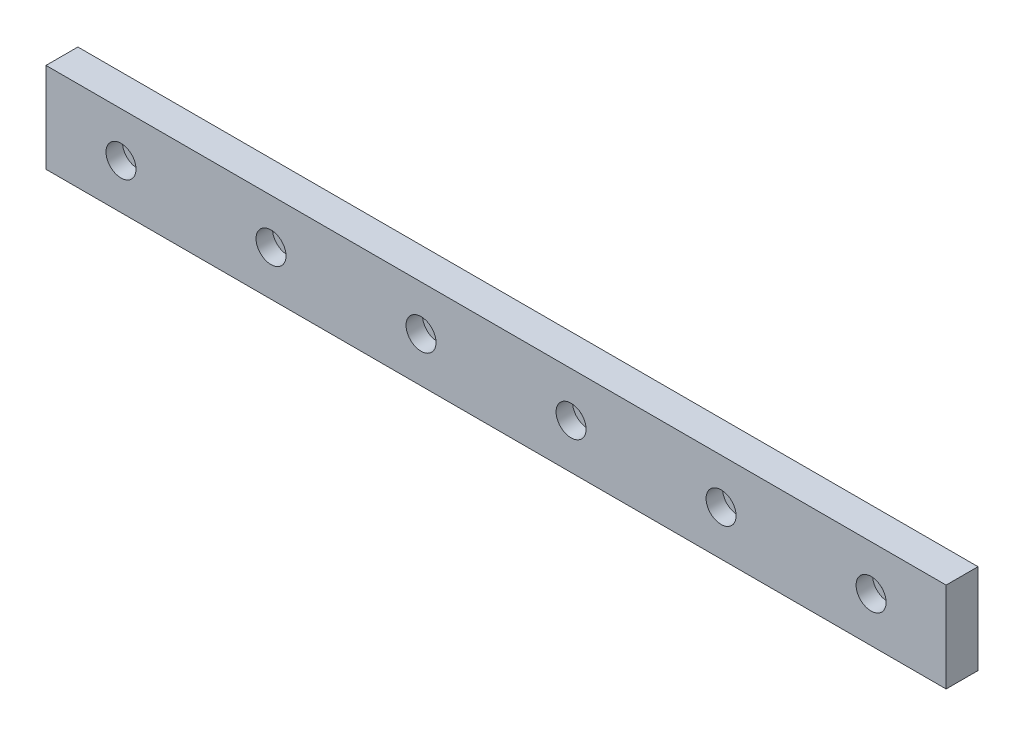
from build123d import *

# Parameters (mm, degrees)
SKETCH1_W                                           = 240
SKETCH1_H                                           = 24
BOSS_EXTRUDE1_DEPTH                                 = 8.5
CBORE_FOR_M4_HEX_SOCKET_HEAD_CAP_SCREW1_D           = 4.5
CBORE_FOR_M4_HEX_SOCKET_HEAD_CAP_SCREW1_CBORE_D     = 8
CBORE_FOR_M4_HEX_SOCKET_HEAD_CAP_SCREW1_CBORE_DEPTH = 4.4
LPATTERN1_COUNT                                     = 6
LPATTERN1_PITCH                                     = 40


with BuildPart() as part:
    # Sketch1 → Boss-Extrude1 (new body)
    with BuildSketch(Plane.XY):
        Rectangle(SKETCH1_W, SKETCH1_H)
    extrude(amount=BOSS_EXTRUDE1_DEPTH)

    # CBORE for M4 Hex Socket Head Cap Screw1 (through all)
    with Locations(Plane.XY.offset(8.5)):
        with Locations((-100, 0)):
            cbore_for_m4_hex_socket_head_cap_screw1 = CounterBoreHole(CBORE_FOR_M4_HEX_SOCKET_HEAD_CAP_SCREW1_D / 2, CBORE_FOR_M4_HEX_SOCKET_HEAD_CAP_SCREW1_CBORE_D / 2, CBORE_FOR_M4_HEX_SOCKET_HEAD_CAP_SCREW1_CBORE_DEPTH)

    # LPattern1: CBORE for M4 Hex Socket Head Cap Screw1 ×6
    with Locations(*[(i * LPATTERN1_PITCH, 0, 0) for i in range(1, LPATTERN1_COUNT)]):
        add(cbore_for_m4_hex_socket_head_cap_screw1, mode=Mode.SUBTRACT)


solid = part.part
